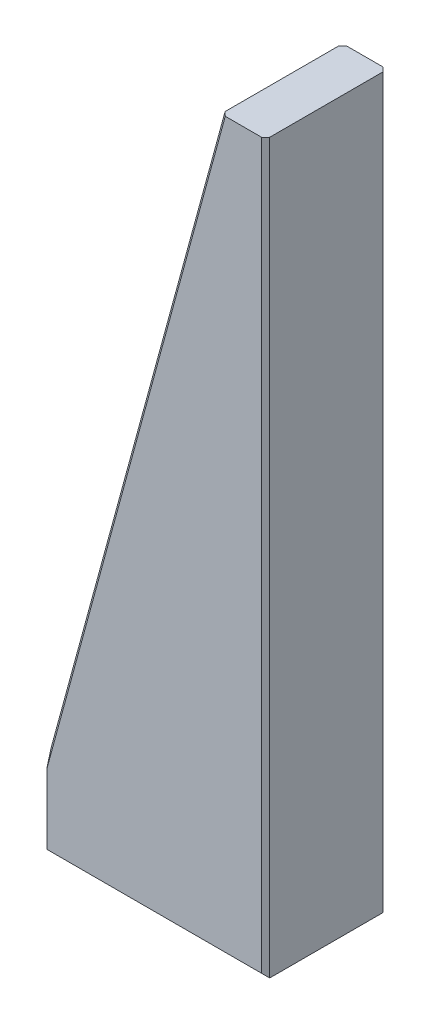
from build123d import *

# Parameters (mm, degrees)
EXTRUDE_1_DEPTH     = 15
CHAMFER_1_SIZE      = 0.5
SKETCH_7_W          = 5.5
SKETCH_7_H          = 20.166666667
SKETCH_7_W_2        = 3
SKETCH_7_H_2        = 20
CUT_EXTRUDE_1_DEPTH = 116


with BuildPart() as part:
    # 草图1 → 凸台-拉伸1 (new body)
    with BuildSketch(Plane.XY):
        Polygon((0, 0), (30, 0), (30, 110), align=None)
    extrude(amount=EXTRUDE_1_DEPTH)

    # 倒角1
    chamfer_1_edges = [part.edges().sort_by_distance(p)[0] for p in [
        (30, 55, 15),
        (30, 55, 0),
        (15, 55, 15),
        (15, 0, 0),
        (15, 55, 0),
        (15, 0, 15),
    ]]
    chamfer(chamfer_1_edges, length=CHAMFER_1_SIZE)

    # 草图7 → 切除-拉伸1 (cut, through all)
    with BuildSketch(Plane.XY.offset(15)):
        with Locations((27.25, 99.916666666)):
            Rectangle(SKETCH_7_W, SKETCH_7_H)
        with Locations((1.5, 10)):
            Rectangle(SKETCH_7_W_2, SKETCH_7_H_2)
    extrude(amount=-CUT_EXTRUDE_1_DEPTH, mode=Mode.SUBTRACT)


solid = part.part
